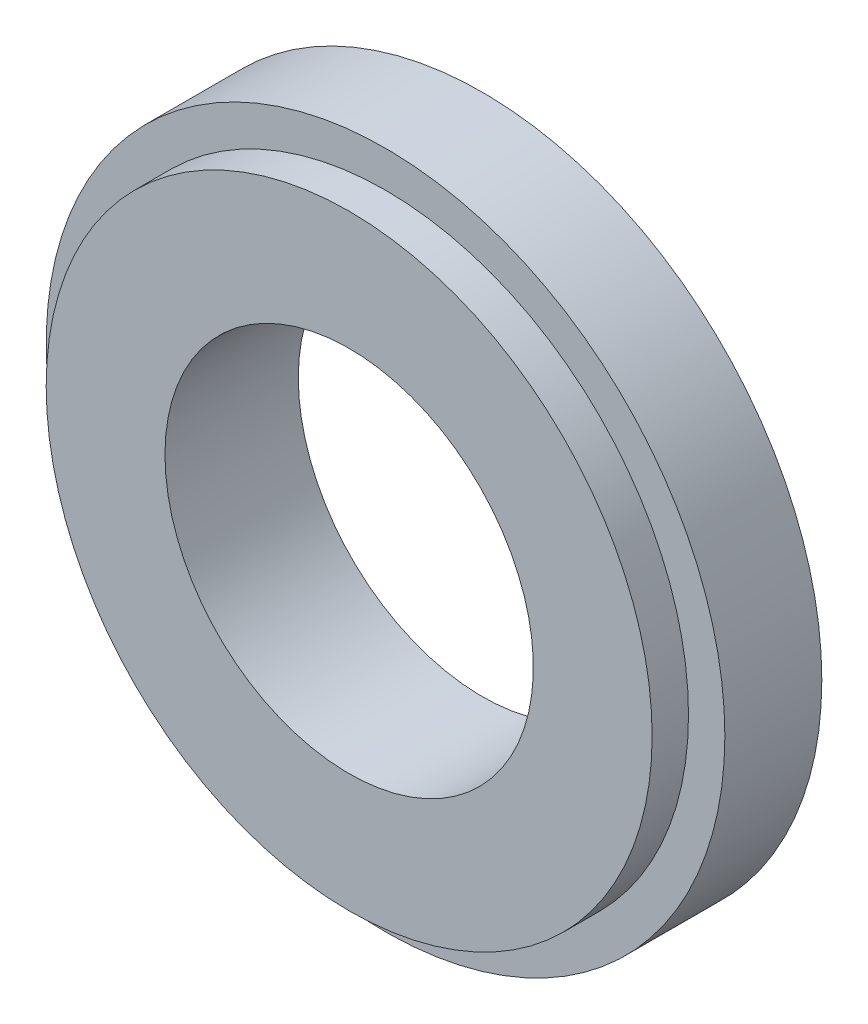
from build123d import *

# Parameters (mm, degrees)
SKETCH1_R           = 28
BOSS_EXTRUDE1_DEPTH = 8
SKETCH2_R           = 25
BOSS_EXTRUDE2_DEPTH = 3
SKETCH4_R           = 15.198536116
CUT_EXTRUDE1_DEPTH  = 42.097445176


with BuildPart() as part:
    # Sketch1 → Boss-Extrude1 (new body)
    with BuildSketch(Plane.XY):
        Circle(SKETCH1_R)
    extrude(amount=BOSS_EXTRUDE1_DEPTH)

    # Sketch2 → Boss-Extrude2 (add)
    with BuildSketch(Plane.XY.offset(8)):
        Circle(SKETCH2_R)
    extrude(amount=BOSS_EXTRUDE2_DEPTH)

    # Sketch4 → Cut-Extrude1 (cut, through all)
    with BuildSketch(Plane(origin=(0, 0, 0), x_dir=(-1, 0, 0), z_dir=(0, 0, -1))):
        Circle(SKETCH4_R)
    extrude(amount=-CUT_EXTRUDE1_DEPTH, mode=Mode.SUBTRACT)


solid = part.part
